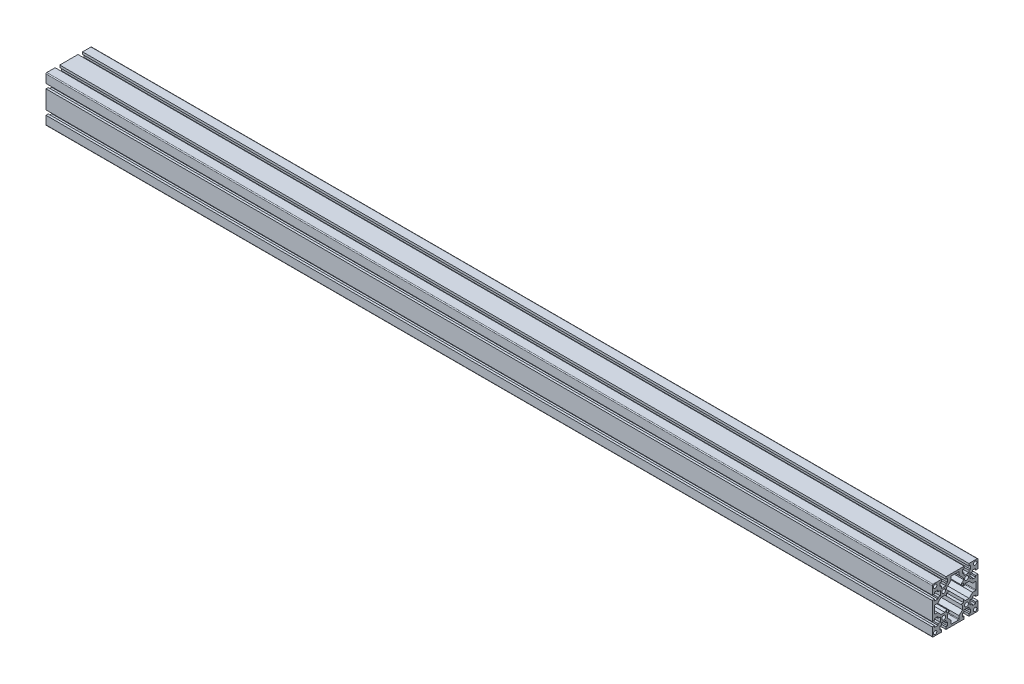
SolidWorks part; units mm, degrees
ref_plane "Front Plane" through (0, 0, 0) normal (0, 0, 1) x (1, 0, 0)
ref_plane "Top Plane" through (0, 0, 0) normal (0, 1, 0) x (1, 0, 0)
ref_plane "Right Plane" through (0, 0, 0) normal (1, 0, 0) x (0, 0, -1)
sketch "草图1" plane through (0, 0, 0) normal (0, 0, 1) x (1, 0, 0)
  line L0 (-530.3448, 0) -> (1019.6552, 0)
  dimension "D1" = 1550
other "Aluminium profile 80 X 80G X R1.5(1)"
ref_plane "Plane2" through (-530.3448, 0, 0) normal (1, 0, 0) x (0, 1, 0)
sketch "Sketch1" plane through (-530.3448, 0, 0) normal (1, 0, 0) x (0, 1, 0)
  line L0 (0, 40) -> (0, 0) construction
  line L1 (0, 0) -> (40, 0) construction
  line L2 (-24.05, 40) -> (-24.05, 36)
  line L3 (-38.5, 40) -> (-24.05, 40)
  line L4 (-40, 38.5) -> (-40, 24.05)
  line L5 (-38.5, -40) -> (-24.05, -40)
  line L6 (40, 38.5) -> (40, 24.05)
  line L7 (-24.05, 36) -> (-26.75, 36)
  line L8 (-26.75, 36) -> (-26.75, 30)
  line L9 (-26.75, 30) -> (-24.05, 30)
  line L10 (-24.05, 30) -> (-24.05, 26)
  line L11 (-24.05, 26) -> (-15.95, 26)
  line L12 (-15.95, 26) -> (-15.95, 30)
  line L13 (-15.95, 30) -> (-13.25, 30)
  line L14 (-13.25, 30) -> (-13.25, 36)
  line L15 (-13.25, 36) -> (-15.95, 36)
  line L16 (-15.95, 36) -> (-15.95, 40)
  line L17 (-40, 15.95) -> (-36, 15.95)
  line L18 (-36, 15.95) -> (-36, 13.25)
  line L19 (-15.95, 40) -> (15.95, 40)
  line L20 (-20, 20) -> (-20, 40) construction
  line L21 (20, 20) -> (20, 40) construction
  line L22 (15.95, 36) -> (15.95, 40)
  line L23 (13.25, 36) -> (15.95, 36)
  line L24 (13.25, 30) -> (13.25, 36)
  line L25 (15.95, 30) -> (13.25, 30)
  line L26 (-36, 13.25) -> (-30, 13.25)
  line L27 (-30, 13.25) -> (-30, 15.95)
  line L28 (-26, 15.95) -> (-26, 24.05)
  line L29 (-26, 24.05) -> (-30, 24.05)
  line L30 (-30, 24.05) -> (-30, 26.75)
  line L31 (-30, 26.75) -> (-36, 26.75)
  line L32 (-36, 26.75) -> (-36, 24.05)
  line L33 (-36, 24.05) -> (-40, 24.05)
  line L34 (-30, 15.95) -> (-26, 15.95)
  line L35 (15.95, 26) -> (15.95, 30)
  line L36 (24.05, 26) -> (15.95, 26)
  line L37 (24.05, 30) -> (24.05, 26)
  line L38 (26.75, 30) -> (24.05, 30)
  line L39 (26.75, 36) -> (26.75, 30)
  line L40 (24.05, 36) -> (26.75, 36)
  line L41 (24.05, 40) -> (24.05, 36)
  line L42 (24.05, -40) -> (24.05, -36)
  line L43 (24.05, -36) -> (26.75, -36)
  line L44 (26.75, -36) -> (26.75, -30)
  line L45 (26.75, -30) -> (24.05, -30)
  line L46 (24.05, -30) -> (24.05, -26)
  line L47 (24.05, -26) -> (15.95, -26)
  line L48 (15.95, -26) -> (15.95, -30)
  line L49 (15.95, -30) -> (13.25, -30)
  line L50 (13.25, -30) -> (13.25, -36)
  line L51 (13.25, -36) -> (15.95, -36)
  line L52 (15.95, -36) -> (15.95, -40)
  line L53 (-15.95, -36) -> (-15.95, -40)
  line L54 (-13.25, -36) -> (-15.95, -36)
  line L55 (-13.25, -30) -> (-13.25, -36)
  line L56 (-15.95, -30) -> (-13.25, -30)
  line L57 (-15.95, -26) -> (-15.95, -30)
  line L58 (-24.05, -26) -> (-15.95, -26)
  line L59 (-24.05, -30) -> (-24.05, -26)
  line L60 (-26.75, -30) -> (-24.05, -30)
  line L61 (-26.75, -36) -> (-26.75, -30)
  line L62 (-24.05, -36) -> (-26.75, -36)
  line L63 (-24.05, -40) -> (-24.05, -36)
  line L64 (-30, -15.95) -> (-26, -15.95)
  line L65 (-36, -26.75) -> (-36, -24.05)
  line L66 (-30, -26.75) -> (-36, -26.75)
  line L67 (-30, -24.05) -> (-30, -26.75)
  line L68 (-26, -24.05) -> (-30, -24.05)
  line L69 (-26, -15.95) -> (-26, -24.05)
  line L70 (-30, -13.25) -> (-30, -15.95)
  line L71 (-36, -13.25) -> (-30, -13.25)
  line L72 (-36, -15.95) -> (-36, -13.25)
  line L73 (36, 24.05) -> (40, 24.05)
  line L74 (40, 15.95) -> (36, 15.95)
  line L75 (36, -15.95) -> (36, -13.25)
  line L76 (36, -13.25) -> (30, -13.25)
  line L77 (30, -13.25) -> (30, -15.95)
  line L78 (26, -15.95) -> (26, -24.05)
  line L79 (26, -24.05) -> (30, -24.05)
  line L80 (30, -24.05) -> (30, -26.75)
  line L81 (30, -26.75) -> (36, -26.75)
  line L82 (36, -26.75) -> (36, -24.05)
  line L83 (30, -15.95) -> (26, -15.95)
  line L84 (30, 15.95) -> (26, 15.95)
  line L85 (36, 26.75) -> (36, 24.05)
  line L86 (30, 26.75) -> (36, 26.75)
  line L87 (30, 24.05) -> (30, 26.75)
  line L88 (26, 24.05) -> (30, 24.05)
  line L89 (26, 15.95) -> (26, 24.05)
  line L90 (30, 13.25) -> (30, 15.95)
  line L91 (36, 13.25) -> (30, 13.25)
  line L92 (36, 15.95) -> (36, 13.25)
  line L93 (-36, -15.95) -> (-40, -15.95)
  line L94 (-36, -24.05) -> (-40, -24.05)
  line L95 (36, -15.95) -> (40, -15.95)
  line L96 (36, -24.05) -> (40, -24.05)
  line L97 (-13, 18) -> (-10, 15)
  line L98 (-15, 15) -> (-10, 15)
  line L99 (-15, 15) -> (-15, 10)
  line L100 (-15, -15) -> (-10, -15)
  line L101 (15, 15) -> (15, 10)
  line L102 (-18, 13) -> (-15, 10)
  line L104 (13, 18) -> (10, 15)
  line L105 (13, -18) -> (10, -15)
  line L106 (20, -15) -> (15, -10)
  line L107 (-18, -13) -> (-15, -10)
  line L108 (-13, -18) -> (-10, -15)
  line L109 (15, -10) -> (15, -15)
  line L110 (10, 15) -> (15, 15)
  line L111 (-15, -10) -> (-15, -15)
  line L112 (10, -15) -> (15, -15)
  line L113 (15, 10) -> (20, 15)
  line L235 (24.05, 40) -> (38.5, 40)
  line L249 (-40, 15.95) -> (-40, -15.95)
  line L250 (-20, 20) -> (-26, 20) construction
  line L264 (40, 15.95) -> (40, -15.95)
  line L265 (-13, 24.5) -> (-7, 30.5)
  line L266 (-7, 30.5) -> (-7, 35.5)
  line L267 (7, 35.5) -> (7, 30.5)
  line L268 (7, 30.5) -> (13, 24.5)
  line L269 (-6, -36.5) -> (6, -36.5)
  line L270 (-13, 24.5) -> (-13, 18)
  line L271 (-35.5, 7) -> (-30.5, 7)
  line L272 (-30.5, 7) -> (-24.5, 13)
  line L273 (-24.5, 13) -> (-18, 13)
  line L274 (13, 24.5) -> (13, 18)
  line L275 (-15.95, -40) -> (15.95, -40)
  line L276 (35.5, 7) -> (30.5, 7)
  line L277 (30.5, 7) -> (22.5, 15)
  line L278 (24.05, -40) -> (38.5, -40)
  line L279 (20, 15) -> (22.5, 15)
  line L333 (-13, -24.5) -> (-13, -18)
  line L336 (-13, -24.5) -> (-7, -30.5)
  line L385 (-7, -30.5) -> (-7, -35.5)
  line L386 (-36.5, 6) -> (-36.5, -6)
  line L387 (7, -35.5) -> (7, -30.5)
  line L429 (7, -30.5) -> (13, -24.5)
  line L430 (13, -24.5) -> (13, -18)
  line L494 (20, -15) -> (22.5, -15)
  line L496 (30.5, -7) -> (22.5, -15)
  line L497 (35.5, -7) -> (30.5, -7)
  line L498 (-24.5, -13) -> (-18, -13)
  line L499 (-30.5, -7) -> (-24.5, -13)
  line L500 (-35.5, -7) -> (-30.5, -7)
  line L512 (40, -24.05) -> (40, -38.5)
  line L519 (-40, -24.05) -> (-40, -38.5)
  line L520 (-6, 36.5) -> (6, 36.5)
  line L523 (36.5, 6) -> (36.5, -6)
  circle A0 centre (-20, 20) radius 3.4
  circle A2 centre (20, 20) radius 3.4
  circle A3 centre (20, -20) radius 3.4
  circle A7 centre (-20, -20) radius 3.4
  arc A8 (-38.5, 40) -> (-40, 38.5) centre (-38.5, 38.5) ccw
  arc A9 (-40, -38.5) -> (-38.5, -40) centre (-38.5, -38.5) ccw
  arc A10 (38.5, -40) -> (40, -38.5) centre (38.5, -38.5) ccw
  arc A11 (38.5, 40) -> (40, 38.5) centre (38.5, 38.5) cw
  circle A12 centre (-35, 35) radius 3
  circle A13 centre (35, 35) radius 3
  circle A14 centre (35, -35) radius 3
  arc A15 (-6, 36.5) -> (-7, 35.5) centre (-6, 35.5) ccw
  arc A16 (6, 36.5) -> (7, 35.5) centre (6, 35.5) cw
  arc A17 (-36.5, 6) -> (-35.5, 7) centre (-35.5, 6) cw
  arc A18 (-36.5, -6) -> (-35.5, -7) centre (-35.5, -6) ccw
  arc A19 (36.5, -6) -> (35.5, -7) centre (35.5, -6) cw
  arc A20 (36.5, 6) -> (35.5, 7) centre (35.5, 6) ccw
  arc A21 (6, -36.5) -> (7, -35.5) centre (6, -35.5) ccw
  arc A22 (-6, -36.5) -> (-7, -35.5) centre (-6, -35.5) cw
  point P48 (-20, 20)
  point P97 (0, 0)
  point P104 (-7, 36.5)
  point P185 (40, 40)
  point P187 (40, -40)
  point P188 (-40, -40)
  point P190 (-40, 40)
  dimension "D1" = 80
  dimension "D2" = 80
  dimension "D3" = 20
  dimension "D4" = 8.1
  dimension "D5" = 45
  dimension "D6" = 7
  dimension "D7" = 13.5
  dimension "D8" = 6
  dimension "D12" = 5
  dimension "D13" = 5
  dimension "D14" = 20
  dimension "D18" = 1
  dimension "D19" = 14
  dimension "D15" = 6.8
  dimension "D27" = 45
  dimension "D20" = 1.5
  dimension "D11" = 6
  dimension "D9" = 4
  dimension "D10" = 14
  dimension "D16" = 14
  dimension "D17" = 45
  dimension "D21" = 3.5
  dimension "D22" = 3.5
  dimension "D23" = 73
  dimension "D24" = 30
  dimension "D25" = 30
  dimension "D26" = 45
  dimension "D28" = 5
sketch "Sketch10" plane through (1019.6552, 0, 0) normal (1, 0, 0) x (0, 0, -1)
  circle A0 centre (35, -35) radius 3
  circle A1 centre (-35, -35) radius 3 construction
  circle A2 centre (35, 35) radius 3 construction
  dimension "D1" = 6
  dimension "D2" = 70
  dimension "D3" = 70
extrude "Cut-Extrude1" cut sketch "Sketch10" against normal through all
